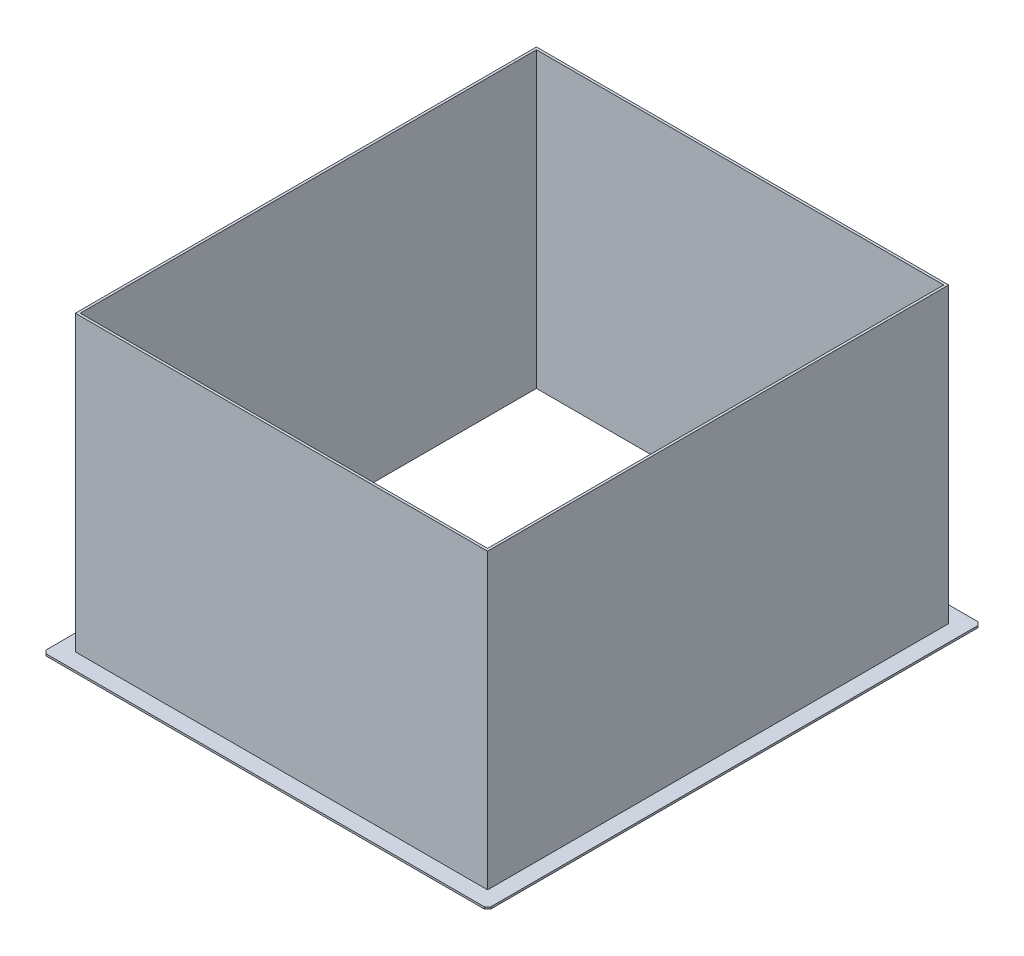
SolidWorks part; units mm, degrees
ref_plane "前视基准面" through (0, 0, 0) normal (0, 0, 1) x (1, 0, 0)
ref_plane "上视基准面" through (0, 0, 0) normal (0, 1, 0) x (1, 0, 0)
ref_plane "右视基准面" through (0, 0, 0) normal (1, 0, 0) x (0, 0, -1)
sketch "草图1" plane through (0, 0, 0) normal (0, 1, 0) x (1, 0, 0)
  line L1 (-125, -140) -> (125, -140)
  line L2 (-125, -140) -> (-125, 140)
  line L3 (-125, 140) -> (125, 140)
  line L4 (125, -140) -> (125, 140)
  line L5 (-125, -140) -> (125, 140) construction
  line L6 (-125, 140) -> (125, -140) construction
  point P0 (0, 0)
  dimension "D1" = 250
  dimension "D2" = 280
extrude "拉伸-薄壁1" add sketch "草图1" along normal blind 180 thin
sketch "草图2" plane through (0, 0, 0) normal (0, -1, 0) x (1, 0, 0)
  line L1 (-126.5, 141.5) -> (126.5, 141.5)
  line L2 (-126.5, 141.5) -> (-126.5, -141.5)
  line L3 (-126.5, -141.5) -> (126.5, -141.5)
  line L4 (126.5, 141.5) -> (126.5, -141.5)
  line L14 (136.5, -151.5) -> (136.5, 151.5)
  line L15 (136.5, 151.5) -> (-136.5, 151.5)
  line L16 (-136.5, 151.5) -> (-136.5, -151.5)
  line L17 (-136.5, -151.5) -> (136.5, -151.5)
  line L18 (136.5, -151.5) -> (136.5, 151.5)
  line L19 (136.5, 151.5) -> (-136.5, 151.5)
  line L20 (-136.5, 151.5) -> (-136.5, -151.5)
  line L21 (-136.5, -151.5) -> (136.5, -151.5)
  dimension "D1" = 10
extrude "凸台-拉伸1" add sketch "草图2" along normal blind 1.2 separate body
chamfer "倒角1" distance 2 angle 45 4 edges at (-136.5, -0.6, 151.5) (-136.5, -0.6, -151.5) (136.5, -0.6, -151.5) (136.5, -0.6, 151.5)
